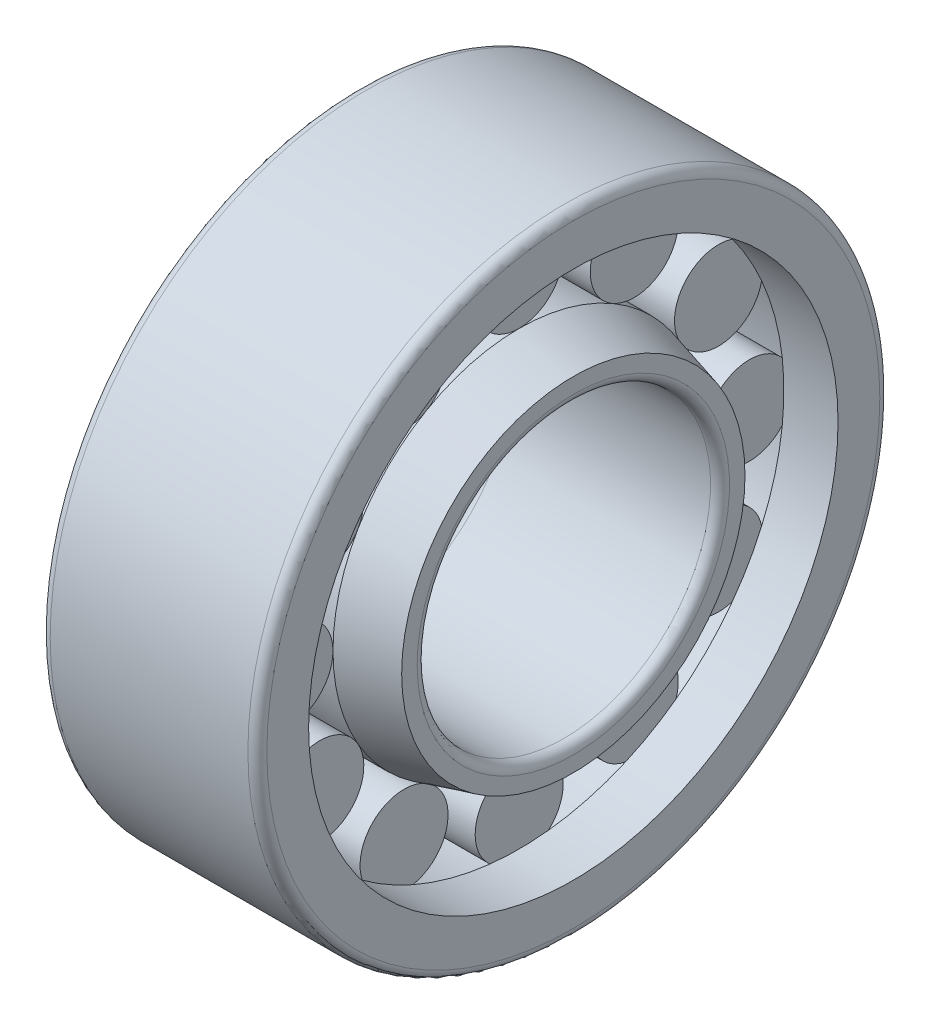
SolidWorks part; units mm, degrees
revolve "Base-Revolve" add sketch "Sketch2" angle 360 about L0
sketch "Sketch2" plane through (0, 0, 0) normal (0, 0, 1) x (1, 0, 0)
  line L0 (-10.0801, 0) -> (21.9267, 0) construction
  line L1 (12, 41.25) -> (36, 41.25)
  line L2 (0, 34.4883) -> (12, 41.25)
  line L3 (0, 34.4883) -> (0, 34.6)
  line L4 (2.1, 32.5) -> (45.9, 32.5)
  line L5 (48, 38.0346) -> (48, 34.6)
  line L7 (48, 38.0346) -> (36, 41.25)
  arc A0 (45.9, 32.5) -> (48, 34.6) centre (45.9, 34.6) ccw
  arc A1 (0, 34.6) -> (2.1, 32.5) centre (2.1, 34.6) ccw
  point P13 (48, 32.5)
  point P16 (0, 32.5)
material "GCr15SiMn"
ref_plane "Plane1" through (0, 0, 0) normal (0, 0, 1) x (1, 0, 0)
ref_plane "Plane2" through (0, 0, 0) normal (0, 1, 0) x (1, 0, 0)
ref_plane "Plane3" through (0, 0, 0) normal (1, 0, 0) x (0, 0, -1)
sketch "Sketch dimensions" plane through (0, 0, 0) normal (0, 0, 1) x (1, 0, 0)
  line L0 (0, 0) -> (2.1, 0)
  line L1 (2.1, 0) -> (4.2, 0)
  line L2 (4.2, 0) -> (52.2, 0)
  line L3 (52.2, 0) -> (117.2, 0)
  line L4 (117.2, 0) -> (199.7, 0)
  line L5 (199.7, 0) -> (339.7, 0)
  line L7 (339.7, 0) -> (461.2, 0)
sketch "Sketch3" plane through (0, 0, 0) normal (0, 0, 1) x (1, 0, 0)
  line L0 (12, 41.25) -> (12, -41.25) construction
  line L1 (36, 41.25) -> (36, -41.25) construction
  line L2 (-1.6039, 51) -> (13.5036, 51) construction
  line L4 (12, 51) -> (36, 51)
  line L5 (12, 51) -> (12, 41.2499)
  line L6 (12, 41.2499) -> (36, 41.2499)
  line L7 (36, 51) -> (36, 41.2499)
revolve "Boss-Revolve1" add sketch "Sketch3" angle 360 about L2
sketch "Sketch4" plane through (0, 0, 0) normal (0, 0, 1) x (1, 0, 0)
  line L0 (0, 0) -> (17.8006, 0) construction
  line L1 (-10.0801, 0) -> (21.9267, 0) construction
  line L2 (36, 58.65) -> (48, 58.65)
  line L3 (2.1, 70) -> (45.9, 70)
  line L4 (0, 67.9) -> (0, 58.65)
  line L5 (0, 58.65) -> (12, 58.65)
  line L6 (48, 67.9) -> (48, 58.65)
  line L7 (12, 60.75) -> (36, 60.75)
  line L8 (12, 60.75) -> (12, 58.65)
  line L10 (36, 60.75) -> (36, 58.65)
  arc A0 (45.9, 70) -> (48, 67.9) centre (45.9, 67.9) cw
  arc A1 (2.1, 70) -> (0, 67.9) centre (2.1, 67.9) ccw
  point P15 (48, 70)
  point P18 (0, 70)
revolve "Boss-Revolve2" add sketch "Sketch4" angle 360 about L0
pattern_circular "CirPattern1" count 12 over 360 about axis through (0, 0, 0) along (1, 0, 0) of "Boss-Revolve1"
equation "\"DD@Sketch2\" = \"内径@Sketch dimensions\""
equation "\"FW@Sketch2\" = \"参考FW@Sketch dimensions\""
equation "\"D1@Sketch2\" = \"倒角小@Sketch dimensions\""
equation "\"EW@Sketch4\" = \"参考EW@Sketch dimensions\""
equation "\"D@Sketch4\" = \"外径@Sketch dimensions\""
equation "\"D2@Sketch4\" = \"倒角大@Sketch dimensions\""
equation "\"B@Sketch4\" = \"宽度@Sketch dimensions\""
equation "\"D1@Sketch3\" =  ( \"EW@Sketch4\" - \"FW@Sketch2\" )  / 4 + \"FW@Sketch2\" / 2"
equation "\"D2@Sketch3\" =  0.25*( \"EW@Sketch4\" - \"FW@Sketch2\" ) +0.0001"
equation "\"D2@Sketch2\" = \"B@Sketch4\""
equation "\"D4@Sketch2\" = \"FW@Sketch2\" + 4 *\"D1@Sketch2\""
equation "\"滚珠位置@Sketch2\" = \"D2@Sketch2\"/4"
equation "\"D3@Sketch4\" = \"D2@Sketch4\""
equation "\"D1@CirPattern1\" = 0.75*\"D1@Sketch3\" * 3.14 / \"D2@Sketch3\""
